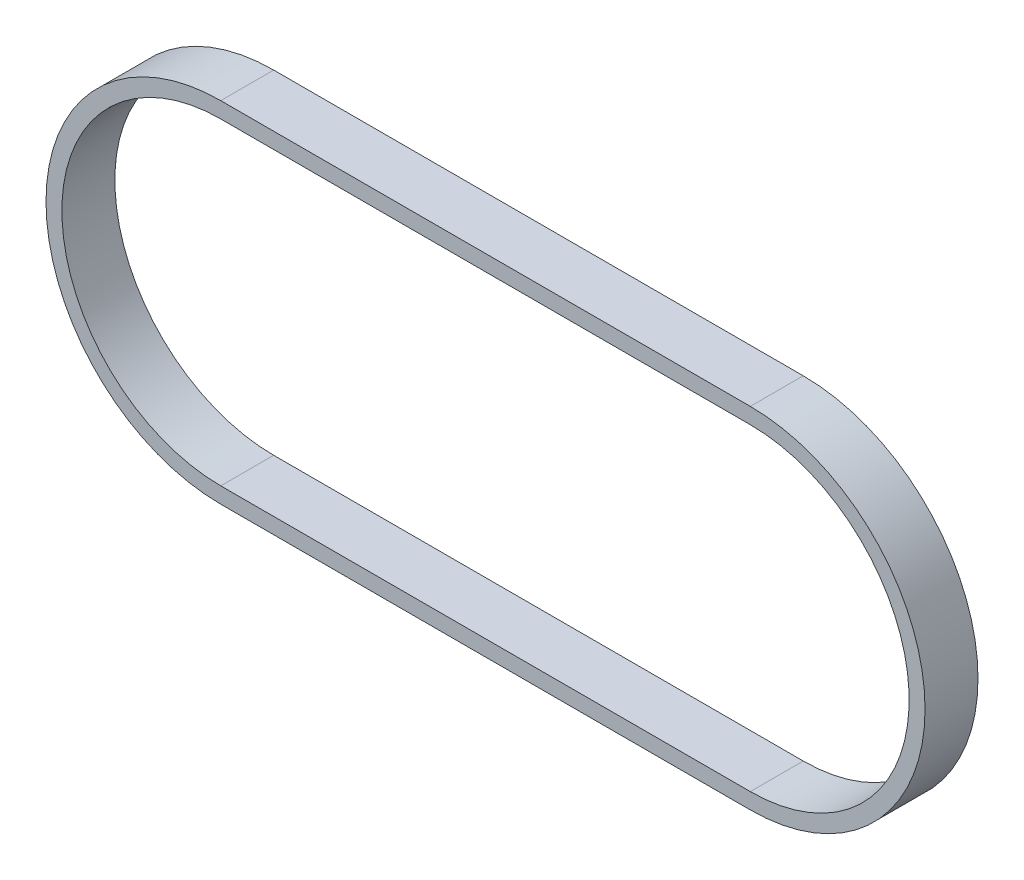
SolidWorks part; units mm, degrees
ref_plane "前视基准面" through (0, 0, 0) normal (0, 0, 1) x (1, 0, 0)
ref_plane "上视基准面" through (0, 0, 0) normal (0, 1, 0) x (1, 0, 0)
ref_plane "右视基准面" through (0, 0, 0) normal (1, 0, 0) x (0, 0, -1)
other "Configuration Table"
sketch "草图1" plane through (0, 0, 0) normal (0, 0, 1) x (1, 0, 0)
  line L0 (-50, 33) -> (50, 33)
  line L1 (50, -33) -> (-50, -33)
  line L2 (-50, 30) -> (50, 30)
  line L3 (50, -30) -> (-50, -30)
  arc A0 (50, 33) -> (50, -33) centre (50, 0) cw
  arc A1 (-50, -33) -> (-50, 33) centre (-50, 0) cw
  arc A2 (50, 30) -> (50, -30) centre (50, 0) cw
  arc A3 (-50, -30) -> (-50, 30) centre (-50, 0) cw
  point P0 (0, 0)
  dimension "D1" = 33
  dimension "D2" = 30
  dimension "D3" = 50
  dimension "D4" = 100
extrude "凸台-拉伸1" add sketch "草图1" against normal mid plane 10
